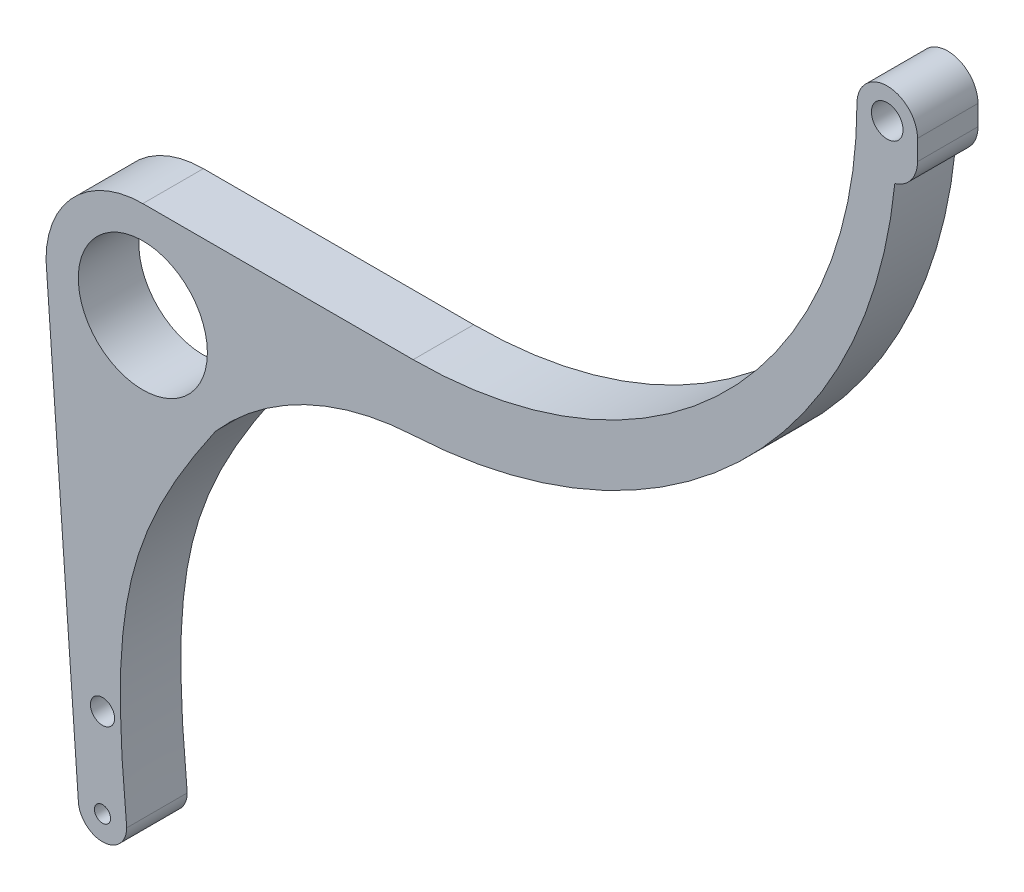
from build123d import *

# Parameters (mm, degrees)
SKETCH_1_R      = 2
SKETCH_1_R_2    = 16
SKETCH_1_R_3    = 3.91899873
SKETCH_1_R_4    = 3
EXTRUDE_1_DEPTH = 15


with BuildPart() as part:
    # 草图1 → 凸台-拉伸1 (new body)
    with BuildSketch(Plane.XY):
        with BuildLine():
            Line((-14, 112), (-6, 0))
            ThreePointArc((-6, 0), (0, -6), (6, 0))
            add(Edge.make_bspline(
                [(6, 0), (1.588652615, 45.680929706), (5.604102499, 63.643200211), (28.004797731, 96.13093391)],
                knots=[0, 0, 0, 0, 0.788155359, 0.788155359, 0.788155359, 0.788155359], degree=3))
            ThreePointArc((28.004797731, 96.13093391), (50.113637924, 112.900750568), (77, 119.767416406))
            ThreePointArc((77, 119.767416406), (157.787149523, 154.485384951), (196.379869136, 233.494896157))
            ThreePointArc((196.379869136, 233.494896157), (200.439238403, 236.311917913), (202, 241))
            Line((202, 241), (202, 246))
            ThreePointArc((202, 246), (194.5, 253.5), (187, 246))
            ThreePointArc((187, 246), (154.781745931, 168.218254069), (77, 136))
            Line((77, 136), (10, 136))
            ThreePointArc((10, 136), (-6.970562748, 128.970562748), (-14, 112))
        make_face()
        Circle(SKETCH_1_R, mode=Mode.SUBTRACT)
        with Locations((10, 112)):
            Circle(SKETCH_1_R_2, mode=Mode.SUBTRACT)
        with Locations((194.5, 246)):
            Circle(SKETCH_1_R_3, mode=Mode.SUBTRACT)
        with Locations((0, 22)):
            Circle(SKETCH_1_R_4, mode=Mode.SUBTRACT)
    extrude(amount=EXTRUDE_1_DEPTH)


solid = part.part
